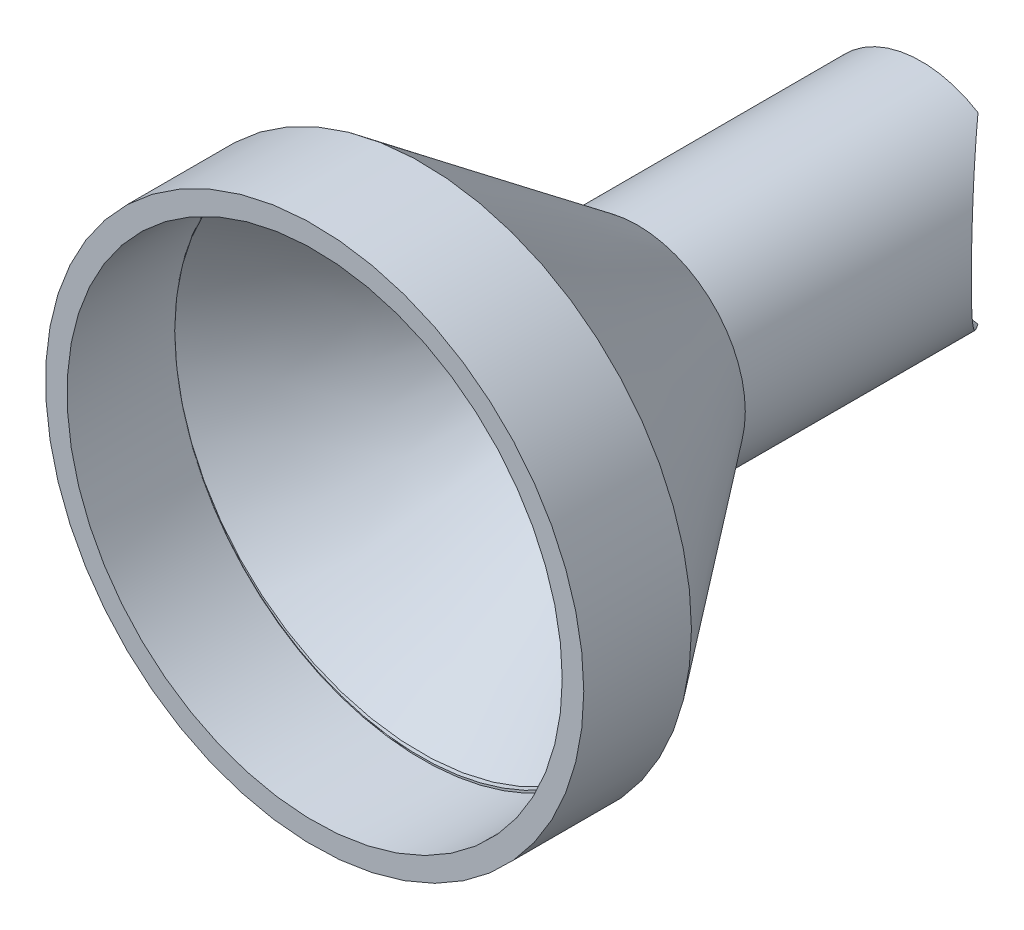
from build123d import *

# Parameters (mm, degrees)
SKETCH_1_R          = 25.000000000000025
SKETCH_1_R_2        = 23.00000000000003
EXTRUDE_1_DEPTH     = 10
SKETCH_2_R          = 10
SKETCH_2_R_2        = 8
EXTRUDE_2_DEPTH     = 10
SKETCH_5_R          = 10
SKETCH_5_R_2        = 8
EXTRUDE_3_DEPTH     = 60
SKETCH_7_R          = 10.000000000000009
CUT_EXTRUDE_1_DEPTH = 30


with BuildPart() as part:
    # 草图1 → 凸台-拉伸1 (new body)
    with BuildSketch(Plane.XY):
        Circle(SKETCH_1_R)
        Circle(SKETCH_1_R_2, mode=Mode.SUBTRACT)
    extrude(amount=-EXTRUDE_1_DEPTH)



with BuildPart() as body_2:
    # 草图2 → 凸台-拉伸2 (new body)
    with BuildSketch(Plane(origin=(0, 0, -30), x_dir=(-1, 0, 0), z_dir=(0, 0, -1))):
        Circle(SKETCH_2_R)
        Circle(SKETCH_2_R_2, mode=Mode.SUBTRACT)
    extrude(amount=EXTRUDE_2_DEPTH)


with BuildPart() as part_1:
    add(part.part)

    add(body_2.part)  # loft_1 joins it to this body
    # loft up to a face of the part (loft_1)
    loft([Face(Wire([part_1.edges().sort_by_distance((-17.113677648, -18.224215686, -10))[0]])), Face(Wire([part_1.edges().sort_by_distance((6.845471059, -7.289686274, -30))[0]]))])

    # 草图5 → 凸台-拉伸3 (add)
    with BuildSketch(Plane(origin=(0, 0, -40), x_dir=(-1, 0, 0), z_dir=(0, 0, -1))):
        Circle(SKETCH_5_R)
        Circle(SKETCH_5_R_2, mode=Mode.SUBTRACT)
    extrude(amount=EXTRUDE_3_DEPTH)

    # 切除-扫描1: sweep along a path in 草图6
    with BuildLine(Plane(origin=(567.6487610779214, 3.3307e-13, 477.55598041107464), x_dir=(-0.9189626632299163, 0, 0.394344549333929), z_dir=(-1e-16, 1, 0))) as sweep_1_path:
        CenterArc((252.99231689471313, -798.553288549715), 96.02083107326227, 0, 360)
    # 草图7 → 切除-扫描1 (sweep, cut)
    with BuildSketch(Plane(origin=(-49.07172931438322, -6.26e-15, -133.08916371965483), x_dir=(-0.9382541725249339, 0, 0.3459466833770077), z_dir=(-0.3459466833770076, 0, -0.9382541725249338))):
        with Locations((-169.14965286891908, 3.3044e-13)):
            Circle(SKETCH_7_R)
    sweep(path=sweep_1_path.line, mode=Mode.SUBTRACT)


with BuildPart() as sweep_1_piece_1:
    # of the separate pieces the step leaves, piece 1, a body of its own (sweep_1_pieces)
    add(part_1.part.solids().sort_by_distance((25, 0, 0))[0])


with BuildPart() as sweep_1_piece_2:
    # of the separate pieces the step leaves, piece 2, a body of its own (sweep_1_pieces)
    add(part_1.part.solids().sort_by_distance((-10, 0, -75.99060176))[0])


with BuildPart() as cut_extrude_1_tool:
    # 草图9 → 切除-拉伸1 (new, symmetric)
    with BuildSketch(Plane(origin=(567.6487610779214, 3.3307e-13, 477.55598041107464), x_dir=(-0.9189626632299163, 0, 0.394344549333929), z_dir=(-1e-16, 1, 0))):
        Polygon((298.93530182729927, -709.2691688884134), (322.9434794568931, -719.5715395575278), (328.1692822059597, -736.3309694794536), (310.61737349860726, -766.3763892056517), (277.35748759673646, -755.1877218619298), (295.795407688748, -719.5715395575278), align=None)
    extrude(amount=CUT_EXTRUDE_1_DEPTH, both=True)


with BuildPart() as sweep_1_piece_1_1:
    add(sweep_1_piece_1.part)

    # 切除-拉伸1: cut by cut_extrude_1_tool
    add(cut_extrude_1_tool.part, mode=Mode.SUBTRACT)

    # 草图10 → 切除-旋转1 (revolve, cut)
    with BuildSketch(Plane(origin=(0, 0, 0), x_dir=(1, 0, 0), z_dir=(0, 1, 0))):
        Polygon((-23, 10), (-23, 0), (0, 0), (-0.8138721873565125, 54.3336376298419), (-7.9999999999999725, 54.3336376298419), (-7.9999999999999725, 30), align=None)
    revolve(axis=Axis((0, 0, 0), (-0.014977478627436109, 0, -0.9998878312760711)), mode=Mode.SUBTRACT)


with BuildPart() as sweep_1_piece_2_1:
    add(sweep_1_piece_2.part)

    # 切除-拉伸1: cut by cut_extrude_1_tool
    add(cut_extrude_1_tool.part, mode=Mode.SUBTRACT)


solid = sweep_1_piece_1_1.part
